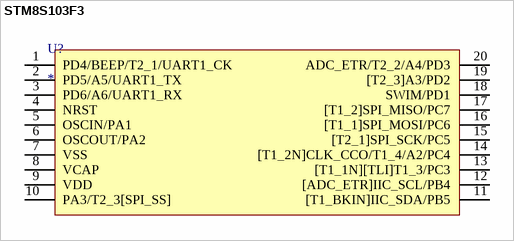
[diagram p0: symbol STM8S103F3]
# Altium schematic symbol library MISC84379-3.SchLib: 1 symbol
Pins are listed as number, name and electrical type; pins without a type are passive.


## STM8S103F3
designator U?
footprint SOP-20 (Footprint not found)
pins: 1 PD4/BEEP/T2_1/UART1_CK, 2 PD5/A5/UART1_TX, 3 PD6/A6/UART1_RX, 4 NRST, 5 OSCIN/PA1, 6 OSCOUT/PA2, 7 VSS, 8 VCAP, 9 VDD, 10 PA3/T2_3[SPI_SS], 11 [T1_BKIN]IIC_SDA/PB5, 12 [ADC_ETR]IIC_SCL/PB4, 13 [T1_1N][TLI]T1_3/PC3, 14 [T1_2N]CLK_CCO/T1_4/A2/PC4, 15 [T2_1]SPI_SCK/PC5, 16 [T1_1]SPI_MOSI/PC6, 17 [T1_2]SPI_MISO/PC7, 18 SWIM/PD1, 19 [T2_3]A3/PD2, 20 ADC_ETR/T2_2/A4/PD3